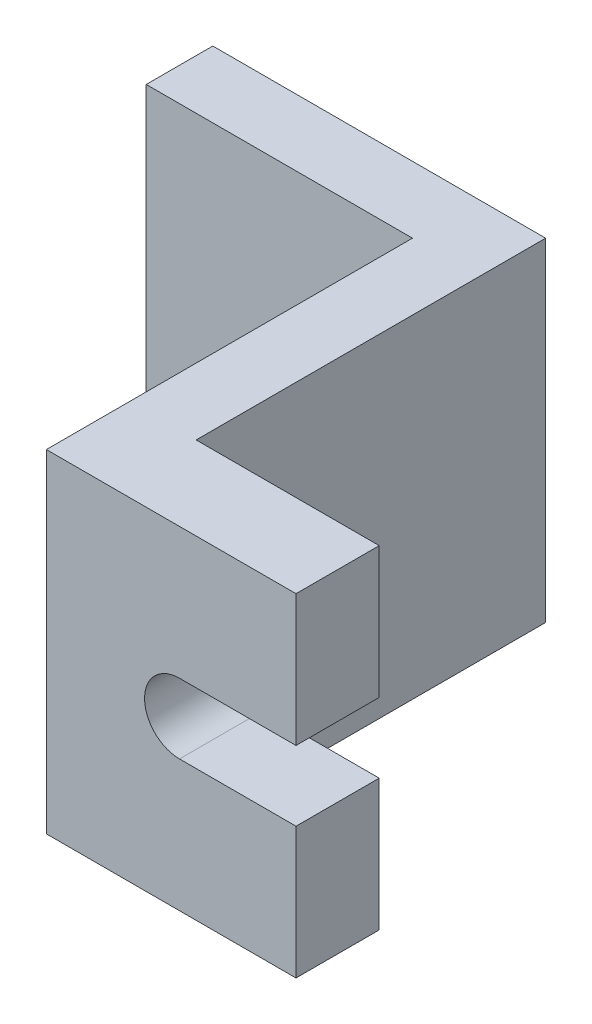
SolidWorks part; units mm, degrees
material "6061 alloy"
ref_plane "Front Plane" through (0, 0, 0) normal (0, 0, 1) x (1, 0, 0)
ref_plane "Top Plane" through (0, 0, 0) normal (0, 1, 0) x (1, 0, 0)
ref_plane "Right Plane" through (0, 0, 0) normal (1, 0, 0) x (0, 0, -1)
sketch "Sketch1" plane through (0, 0, 0) normal (0, 1, 0) x (1, 0, 0)
  line L1 (-22.5743, 8.6535) -> (-2.5743, 8.6535)
  line L2 (-22.5743, 8.6535) -> (-22.5743, 4.6535)
  line L3 (-22.5743, 4.6535) -> (-2.5743, 4.6535)
  line L4 (-2.5743, 8.6535) -> (-2.5743, 4.6535)
  line L5 (-2.5743, 8.6535) -> (-6.5743, 8.6535)
  line L6 (-2.5743, 8.6535) -> (-2.5743, -17.3465)
  line L7 (-2.5743, -17.3465) -> (-6.5743, -17.3465)
  line L8 (-6.5743, 8.6535) -> (-6.5743, -17.3465)
  line L9 (-6.5743, -17.3465) -> (8.4257, -17.3465)
  line L10 (-6.5743, -17.3465) -> (-6.5743, -12.3465)
  line L11 (-6.5743, -12.3465) -> (8.4257, -12.3465)
  line L12 (8.4257, -17.3465) -> (8.4257, -12.3465)
  dimension "D1" = 4
  dimension "D2" = 20
  dimension "D3" = 22
  dimension "D4" = 5
  dimension "D5" = 15
  dimension "D6" = 4
extrude "Boss-Extrude1" add sketch "Sketch1" along normal blind 20 contours L8 L1 L2 L3 | L1 L8 L3 L4 | L8 L11 L6 L3 | L11 L8 L7 L6 | L9 L12 L11 L6
sketch "Sketch2" plane through (0, 0, 12.3465) normal (0, 0, -1) x (-1, 0, 0)
  line L0 (-5.4257, 7.9) -> (-8.8417, 7.9)
  line L3 (-1.4257, 10) -> (-5.4257, 10) construction
  line L4 (-1.4257, 7.9) -> (-5.4257, 7.9)
  line L5 (-1.4257, 12.1) -> (-5.4257, 12.1)
  line L6 (-8.8417, 7.9) -> (-8.8417, 11.8523)
  line L7 (-5.4257, 12.1) -> (-8.8417, 12.1)
  line L8 (-8.8417, 12.1) -> (-8.8417, 11.8523)
  line L10 (2.5743, 20) -> (2.5743, 0) construction
  arc A2 (-1.4257, 7.9) -> (-1.4257, 12.1) centre (-1.4257, 10) ccw
  point P7 (-3.4257, 10)
  dimension "D5" = 2.1
  dimension "D6" = 4
extrude "Cut-Extrude1" cut sketch "Sketch2" against normal blind 15
